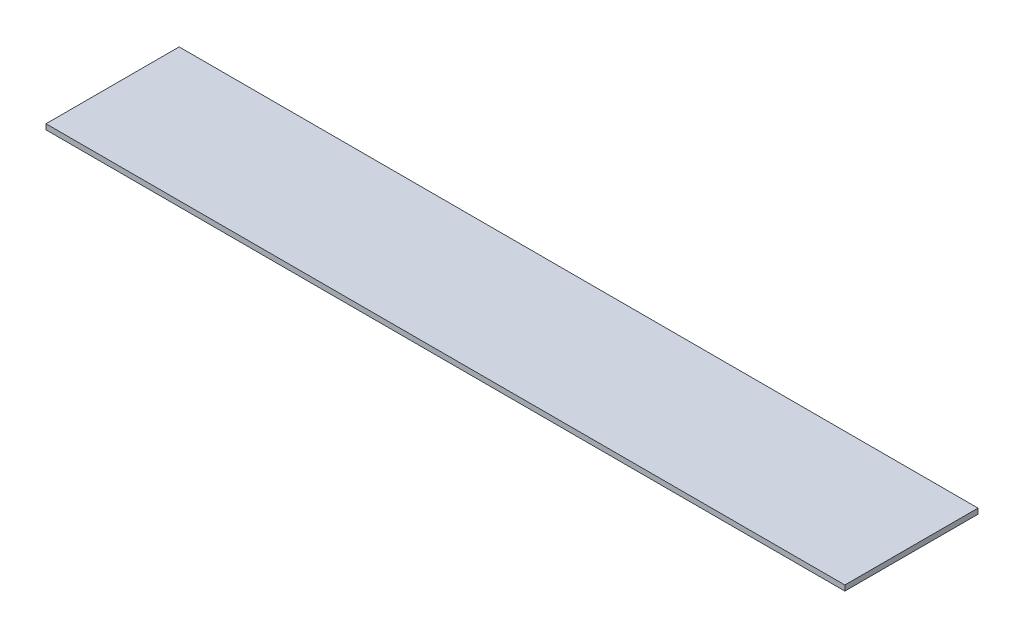
SolidWorks part; units mm, degrees
material "Q235"
ref_plane "前视基准面" through (0, 0, 0) normal (0, 0, 1) x (1, 0, 0)
ref_plane "上视基准面" through (0, 0, 0) normal (0, 1, 0) x (1, 0, 0)
ref_plane "右视基准面" through (0, 0, 0) normal (1, 0, 0) x (0, 0, -1)
sketch "草图1" plane through (0, 0, 0) normal (0, 1, 0) x (1, 0, 0)
  line L1 (0, 0) -> (600, 0)
  line L2 (0, 0) -> (0, 100)
  line L3 (0, 100) -> (600, 100)
  line L4 (600, 0) -> (600, 100)
  dimension "D1" = 600
  dimension "D2" = 100
extrude "凸台-拉伸1" add sketch "草图1" along normal blind 4
